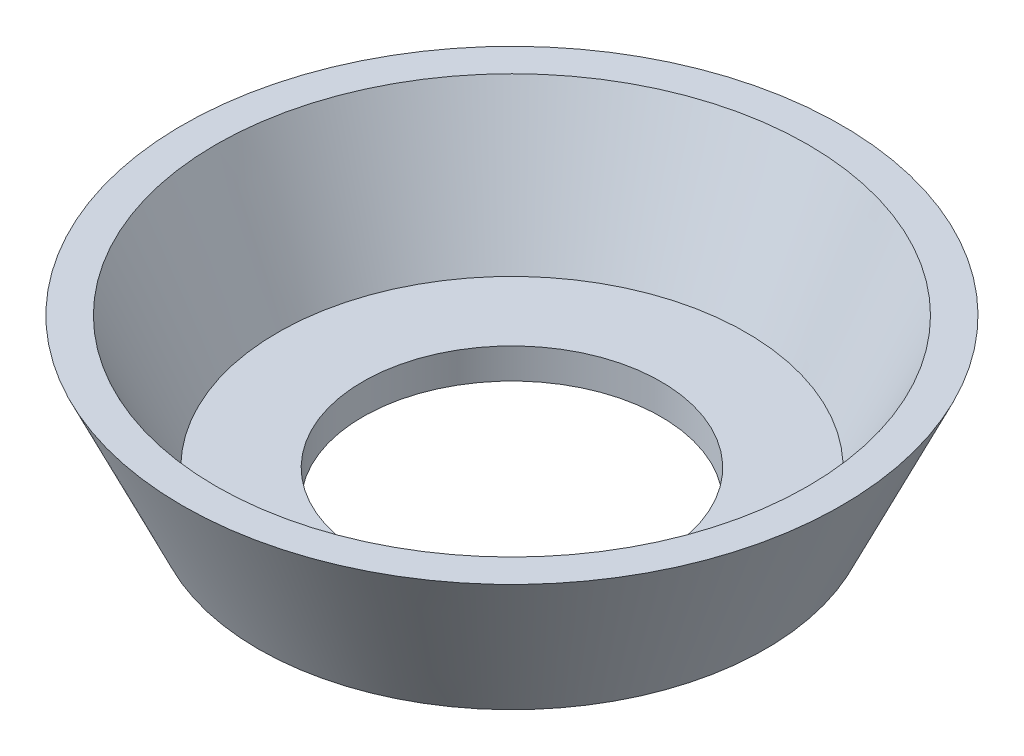
SolidWorks part; units mm, degrees
material "橡胶"
ref_plane "前视" through (0, 0, 0) normal (0, 0, 1) x (1, 0, 0)
ref_plane "上视" through (0, 0, 0) normal (0, 1, 0) x (1, 0, 0)
ref_plane "右视" through (0, 0, 0) normal (1, 0, 0) x (0, 0, -1)
sketch "草图1" plane through (0, 0, 0) normal (0, 0, 1) x (1, 0, 0)
  line L0 (-62.512, 0) -> (69.9761, 0) construction
  line L1 (0, 44.0072) -> (0, -40.8971) construction
  line L2 (-32.5, 16) -> (-25, 0)
  line L3 (-25, 0) -> (-14.7, 0)
  line L4 (-29.1868, 16) -> (-23.093, 3)
  line L5 (-23.093, 3) -> (-14.7, 3)
  line L6 (-32.5, 16) -> (-29.1868, 16)
  line L7 (-14.7, 3) -> (-14.7, 0)
  line L8 (-29.7836, 17.2733) -> (-23.093, 3) construction
  dimension "D1" = 32.5
  dimension "D2" = 25
  dimension "D3" = 14.7
  dimension "D4" = 16
  dimension "D5" = 3
revolve "旋转1" add sketch "草图1" angle 360 about L1
